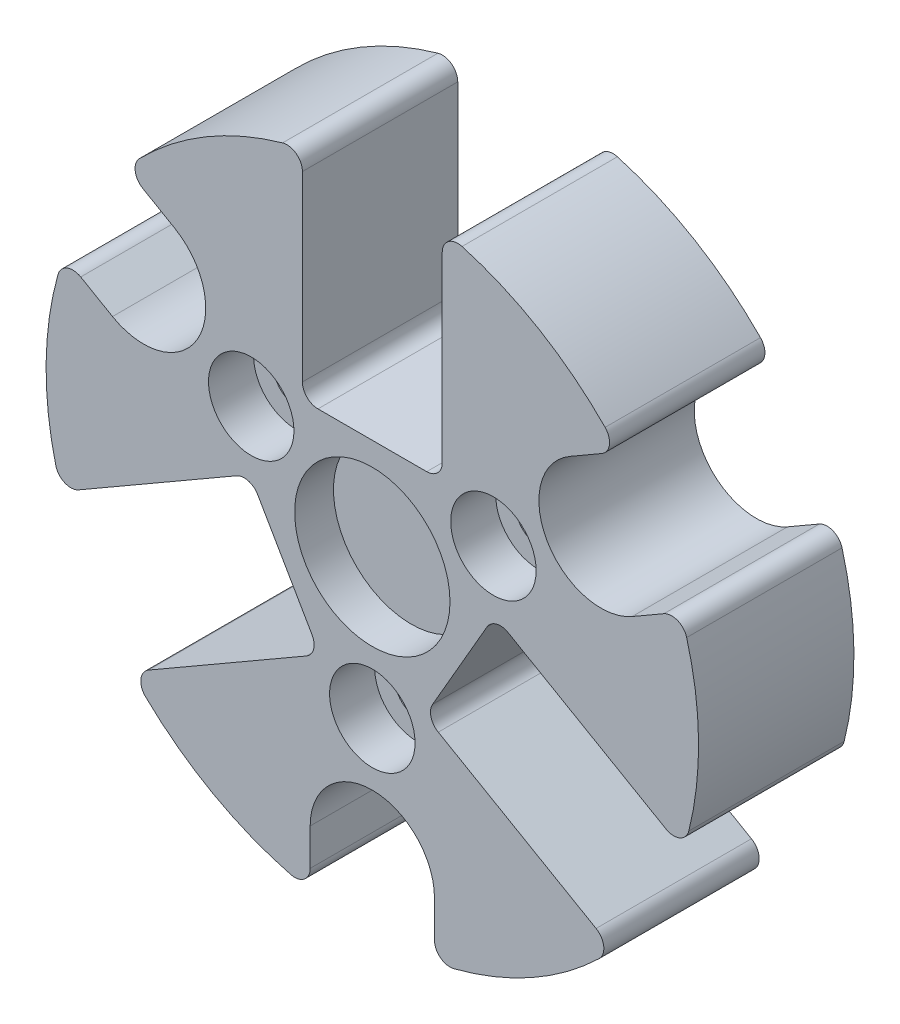
SolidWorks part; units mm, degrees
material "S136"
ref_plane "Front Plane" through (0, 0, 0) normal (0, 0, 1) x (1, 0, 0)
ref_plane "Top Plane" through (0, 0, 0) normal (0, 1, 0) x (1, 0, 0)
ref_plane "Right Plane" through (0, 0, 0) normal (1, 0, 0) x (0, 0, -1)
sketch "Sketch1" plane through (0, 0, 0) normal (0, 0, 1) x (1, 0, 0)
  circle A0 centre (0, 0) radius 21
  dimension "D1" = 42
extrude "Boss-Extrude1" add sketch "Sketch1" along normal blind 10
sketch "Sketch2" plane through (0, 0, 10) normal (0, 0, 1) x (1, 0, 0)
  line L0 (0, 0) -> (0, 12.0641) construction
  line L1 (-4.5, 25.4092) -> (4.5, 25.4092)
  line L2 (-4.5, 25.4092) -> (-4.5, 6.5)
  line L3 (-4.5, 6.5) -> (4.5, 6.5)
  line L4 (4.5, 25.4092) -> (4.5, 6.5)
  dimension "D1" = 9
  dimension "D2" = 6.5
extrude "Cut-Extrude1" cut sketch "Sketch2" against normal blind 12
fillet "Fillet1" radius 1 4 edges at (4.5, 6.5, 5) (-4.5, 6.5, 5) (4.5, 20.5122, 5) (-4.5, 20.5122, 5)
pattern_circular "CirPattern1" count 3 over 360 about axis through (0, 0, 0) along (0, 0, 1) of "Cut-Extrude1", "Fillet1"
hole_wizard "CBORE for M2.5 Hex Socket Head Cap Screw1" positions "Sketch3" profile "Sketch4" counterbore size "M2.5" standard "ISO" end condition through all
sketch "Sketch3" plane through (0, 0, 10) normal (0, 0, 1) x (1, 0, 0)
  point P0 (0, -9)
  dimension "D1" = 9
sketch "Sketch4" plane through (0, -9, 10) normal (1, 0, 0) x (0, -1, 0)
  line L0 (0, 0) -> (0, 10)
  line L1 (0, 10) -> (1.45, 10)
  line L3 (1.45, 10) -> (1.45, 2.9)
  line L4 (1.45, 2.9) -> (2.75, 2.9)
  line L5 (2.75, 2.9) -> (2.75, 0)
  line L7 (2.75, 0) -> (0, 0)
  line L11 (0, -6.35) -> (0, 107.95) construction
  dimension "通孔孔直径" = 2.9
  dimension "通孔孔深度" = 10
  dimension "柱形沉头孔直径" = 5.5
  dimension "柱形沉头孔深度" = 2.9
pattern_circular "CirPattern2" count 3 over 360 about axis through (0, 0, 0) along (0, 0, 1) of "CBORE for M2.5 Hex Socket Head Cap Screw1"
sketch "Sketch5" plane through (0, 0, 10) normal (0, 0, 1) x (1, 0, 0)
  line L0 (0, -17) -> (0, -24.0006) construction
  line L1 (4, -17) -> (4, -24.0006)
  line L2 (-4, -17) -> (-4, -24.0006)
  arc A0 (4, -17) -> (-4, -17) centre (0, -17) ccw
  arc A1 (-4, -24.0006) -> (4, -24.0006) centre (0, -24.0006) ccw
  point P3 (0, -20.5003)
  dimension "D1" = 17
  dimension "D2" = 8
extrude "Cut-Extrude2" cut sketch "Sketch5" against normal through all
fillet "Fillet2" radius 1 2 edges at (4, -20.6155, 5) (-4, -20.6155, 5)
pattern_circular "CirPattern3" count 3 over 360 about axis through (0, 0, 0) along (0, 0, 1) of "Cut-Extrude2", "Fillet2"
sketch "Sketch7" plane through (0, 0, 10) normal (0, 0, 1) x (1, 0, 0)
  circle A0 centre (0, 0) radius 5
  dimension "D1" = 10
extrude "Cut-Extrude4" cut sketch "Sketch7" against normal blind 2.5
